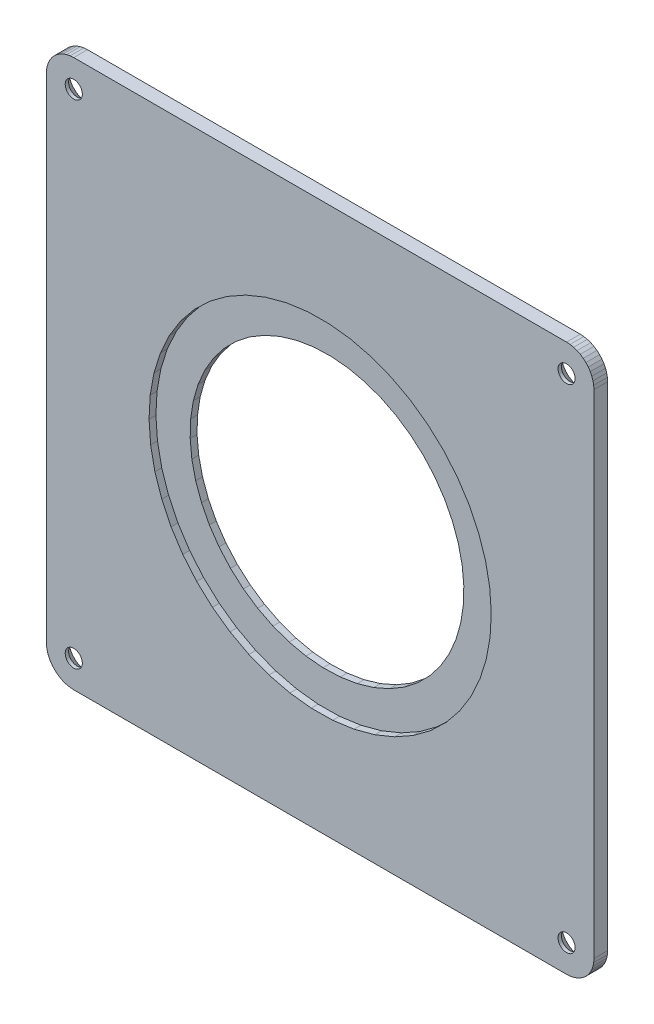
from build123d import *

# Parameters (mm, degrees)
BOSS_EXTRUDE1_DEPTH = 2.000000328
CUT_EXTRUDE1_DEPTH  = 57.60388554
CUT_EXTRUDE2_DEPTH  = 57.60388554
CUT_EXTRUDE3_DEPTH  = 57.60388554
CUT_EXTRUDE4_DEPTH  = 57.60388554
CUT_EXTRUDE5_DEPTH  = 0.999998301
CUT_EXTRUDE6_DEPTH  = 57.577379411
SKETCH9_R           = 2
CUT_EXTRUDE7_DEPTH  = 10
MOVE_FACE1_BY       = 0.75
MOVE_FACE1_2_BY     = 0.75
MOVE_FACE1_3_BY     = 0.75
MOVE_FACE1_4_BY     = 0.75
CHAMFER1_SIZE       = 1.5


with BuildPart() as part:
    # Sketch1 → Boss-Extrude1 (new body)
    with BuildSketch(Plane.XY.offset(37.080600858)):
        Polygon((-39.999999106, -35.99999845), (-39.965778589, -36.522105336), (-39.863705635, -37.035275251), (-39.695519954, -37.530735135), (-39.464101195, -37.999998778), (-39.173413068, -38.43504563), (-38.828425109, -38.828425109), (-38.43504563, -39.173413068), (-37.999998778, -39.464101195), (-37.530735135, -39.695519954), (-37.035275251, -39.863705635), (-36.522105336, -39.965778589), (-35.99999845, -39.999999106), (35.99999845, -39.999999106), (36.522105336, -39.965778589), (37.035275251, -39.863705635), (37.530735135, -39.695519954), (37.999998778, -39.464101195), (38.43504563, -39.173413068), (38.828425109, -38.828425109), (39.173413068, -38.43504563), (39.464101195, -37.999998778), (39.695519954, -37.530735135), (39.863705635, -37.035275251), (39.965778589, -36.522105336), (39.999999106, -35.99999845), (39.999999106, 35.99999845), (39.965778589, 36.522105336), (39.863705635, 37.035275251), (39.695519954, 37.530735135), (39.464101195, 37.999998778), (39.173413068, 38.43504563), (38.828425109, 38.828425109), (38.43504563, 39.173413068), (37.999998778, 39.464101195), (37.530735135, 39.695519954), (37.035275251, 39.863705635), (36.522105336, 39.965778589), (35.99999845, 39.999999106), (-35.99999845, 39.999999106), (-36.522105336, 39.965778589), (-37.035275251, 39.863705635), (-37.530735135, 39.695519954), (-37.999998778, 39.464101195), (-38.43504563, 39.173413068), (-38.828425109, 38.828425109), (-39.173413068, 38.43504563), (-39.464101195, 37.999998778), (-39.695519954, 37.530735135), (-39.863705635, 37.035275251), (-39.965778589, 36.522105336), (-39.999999106, 35.99999845), align=None)
    extrude(amount=-BOSS_EXTRUDE1_DEPTH)

    # Sketch2 → Cut-Extrude1 (cut, through all)
    with BuildSketch(Plane.XY.offset(37.080600858)):
        Polygon((-37.448886782, -36.388229579), (-37.29903698, -36.74999997), (-37.060663104, -37.060663104), (-36.74999997, -37.29903698), (-36.388229579, -37.448886782), (-35.99999845, -37.50000149), (-35.611771047, -37.448886782), (-35.250000656, -37.29903698), (-34.939337522, -37.060663104), (-34.700963646, -36.74999997), (-34.551113844, -36.388229579), (-34.499999136, -35.99999845), (-34.551113844, -35.611771047), (-34.700963646, -35.250000656), (-34.939337522, -34.939337522), (-35.250000656, -34.700963646), (-35.611771047, -34.551113844), (-35.99999845, -34.499999136), (-36.388229579, -34.551113844), (-36.74999997, -34.700963646), (-37.060663104, -34.939337522), (-37.29903698, -35.250000656), (-37.448886782, -35.611771047), (-37.50000149, -35.99999845), align=None)
    extrude(amount=-CUT_EXTRUDE1_DEPTH, mode=Mode.SUBTRACT)

    # Sketch3 → Cut-Extrude2 (cut, through all)
    with BuildSketch(Plane.XY.offset(37.080600858)):
        Polygon((-37.448886782, 35.611771047), (-37.29903698, 35.250000656), (-37.060663104, 34.939337522), (-36.74999997, 34.700963646), (-36.388229579, 34.551113844), (-35.99999845, 34.499999136), (-35.611771047, 34.551113844), (-35.250000656, 34.700963646), (-34.939337522, 34.939337522), (-34.700963646, 35.250000656), (-34.551113844, 35.611771047), (-34.499999136, 35.99999845), (-34.551113844, 36.388229579), (-34.700963646, 36.74999997), (-34.939337522, 37.060663104), (-35.250000656, 37.29903698), (-35.611771047, 37.448886782), (-35.99999845, 37.50000149), (-36.388229579, 37.448886782), (-36.74999997, 37.29903698), (-37.060663104, 37.060663104), (-37.29903698, 36.74999997), (-37.448886782, 36.388229579), (-37.50000149, 35.99999845), align=None)
    extrude(amount=-CUT_EXTRUDE2_DEPTH, mode=Mode.SUBTRACT)

    # Sketch4 → Cut-Extrude3 (cut, through all)
    with BuildSketch(Plane.XY.offset(37.080600858)):
        Polygon((34.787815064, -36.8835181), (35.057790577, -37.167146802), (35.391975194, -37.371244282), (35.767596215, -37.481889129), (35.99999845, -37.48762235), (36.159053327, -37.491546138), (36.539680178, -37.399572712), (36.88352638, -37.212212123), (37.167163198, -36.942245137), (37.371270724, -36.608066656), (37.481926864, -36.232448961), (37.491590859, -35.840992022), (37.399556488, -35.460323095), (37.212185562, -35.116482526), (36.942210048, -34.832850099), (36.608025432, -34.628756344), (36.232404411, -34.518111497), (35.840947181, -34.508455545), (35.460323095, -34.600444138), (35.116482526, -34.787815064), (34.832850099, -35.057790577), (34.628756344, -35.391975194), (34.518111497, -35.767596215), (34.508455545, -36.159053445), (34.600444138, -36.539677531), align=None)
    extrude(amount=-CUT_EXTRUDE3_DEPTH, mode=Mode.SUBTRACT)

    # Sketch5 → Cut-Extrude4 (cut, through all)
    with BuildSketch(Plane(origin=(0, 0, 35.08060053), x_dir=(-1, 0, 0), z_dir=(0, 0, -1))):
        Polygon((-36.388229579, 37.448886782), (-36.74999997, 37.29903698), (-37.060663104, 37.060663104), (-37.29903698, 36.74999997), (-37.448886782, 36.388229579), (-37.50000149, 35.99999845), (-37.448886782, 35.611771047), (-37.29903698, 35.250000656), (-37.060663104, 34.939337522), (-36.74999997, 34.700963646), (-36.388229579, 34.551113844), (-35.99999845, 34.499999136), (-35.611771047, 34.551113844), (-35.250000656, 34.700963646), (-34.939337522, 34.939337522), (-34.700963646, 35.250000656), (-34.551113844, 35.611771047), (-34.499999136, 35.99999845), (-34.551113844, 36.388229579), (-34.700963646, 36.74999997), (-34.939337522, 37.060663104), (-35.250000656, 37.29903698), (-35.611771047, 37.448886782), (-35.99999845, 37.50000149), align=None)
    extrude(amount=-CUT_EXTRUDE4_DEPTH, mode=Mode.SUBTRACT)

    # Sketch6 → Cut-Extrude5 (cut)
    with BuildSketch(Plane.XY.offset(37.080600858)):
        Polygon((-23.146180436, -9.447447956), (-21.779589355, -12.273938395), (-20.069517195, -14.906859957), (-18.042938784, -17.304692417), (-15.731809661, -19.429620355), (-13.172583655, -21.248130128), (-10.405616835, -22.73154445), (-7.474547718, -23.856470361), (-4.425600171, -24.605164304), (-1.306858379, -24.965818971), (1.832493464, -24.932749569), (4.94294567, -24.506473914), (7.975445129, -23.693718016), (10.882166214, -22.507296875), (13.617269695, -20.965922624), (16.137620434, -19.093904644), (18.403470516, -16.920762137), (20.379088819, -14.480772428), (22.033315152, -11.812409386), (23.34006317, -8.957758546), (24.278724566, -5.961838178), (24.834495038, -2.871896373), (24.998612702, 0.263337133), (24.768486619, 3.394417698), (24.147747084, 6.471966393), (23.146180436, 9.447447956), (21.779589355, 12.273938395), (20.069517195, 14.906859957), (18.042938784, 17.304692417), (15.731809661, 19.429620355), (13.172583655, 21.248130128), (10.405616835, 22.73154445), (7.474547718, 23.856470361), (4.425600171, 24.605164304), (1.306858379, 24.965818971), (-1.832493464, 24.932749569), (-4.94294567, 24.506473914), (-7.975445129, 23.693718016), (-10.882166214, 22.507296875), (-13.617269695, 20.965922624), (-16.137620434, 19.093904644), (-18.403470516, 16.920762137), (-20.379088819, 14.480772428), (-22.033315152, 11.812409386), (-23.34006317, 8.957758546), (-24.278724566, 5.961838178), (-24.834495038, 2.871896373), (-24.998612702, -0.263337133), (-24.768486619, -3.394417698), (-24.147747084, -6.471966393), align=None)
    extrude(amount=-CUT_EXTRUDE5_DEPTH, mode=Mode.SUBTRACT)

    # Sketch7 → Cut-Extrude6 (cut, through all)
    with BuildSketch(Plane.XY.offset(36.080602556)):
        Polygon((-19.744809717, -3.184724366), (-19.18996498, -5.634292495), (-18.332481384, -7.995004766), (-17.185883597, -10.229631327), (-15.768256038, -12.302929536), (-14.101952314, -14.182204381), (-12.213253416, -15.837816522), (-10.131943971, -17.243657261), (-7.89084658, -18.377555534), (-5.525306799, -19.221628085), (-3.072628984, -19.762564451), (-0.57149434, -19.991831854), (1.938653179, -19.905818626), (4.418227356, -19.50587891), (6.828122772, -18.79831776), (9.130334482, -17.794296145), (11.28855627, -16.509648412), (13.268750161, -14.964633621), (15.039687976, -13.183617964), (16.573440284, -11.194689199), (17.845820636, -9.029212408), (18.836760893, -6.721339654), (19.530635327, -4.30746749), (19.916500896, -1.825664192), (19.988268614, 0.684931001), (19.744809717, 3.184724366), (19.18996498, 5.634292495), (18.332481384, 7.995004766), (17.185883597, 10.229631327), (15.768256038, 12.302929536), (14.101952314, 14.182204381), (12.213253416, 15.837816522), (10.131943971, 17.243657261), (7.89084658, 18.377555534), (5.525306799, 19.221628085), (3.072628984, 19.762564451), (0.57149434, 19.991831854), (-1.938653179, 19.905818626), (-4.418227356, 19.50587891), (-6.828122772, 18.79831776), (-9.130334482, 17.794296145), (-11.28855627, 16.509648412), (-13.268750161, 14.964633621), (-15.039687976, 13.183617964), (-16.573440284, 11.194689199), (-17.845820636, 9.029212408), (-18.836760893, 6.721339654), (-19.530635327, 4.30746749), (-19.916500896, 1.825664192), (-19.988268614, -0.684931001), align=None)
    extrude(amount=-CUT_EXTRUDE6_DEPTH, mode=Mode.SUBTRACT)

    # Sketch9 → Cut-Extrude7 (cut)
    with BuildSketch(Plane(origin=(0, 0, 35.08060053), x_dir=(-1, 0, 0), z_dir=(0, 0, -1))):
        with Locations((35.99999845, 35.99999845)):
            Circle(SKETCH9_R)
        with Locations(Location((35.99999845, -35.99999845, 0), (0, 0, 180))):
            Circle(SKETCH9_R)
        with Locations((-35.99999845, -35.99999845)):
            Circle(SKETCH9_R)
        with Locations(Location((-35.99999845, 35.99999845, 0), (0, 0, 180))):
            Circle(SKETCH9_R)
    extrude(amount=-CUT_EXTRUDE7_DEPTH, mode=Mode.SUBTRACT)

    # Move Face1: a curved face moved outward by 0.75
    add(Solid.thicken(part.faces().sort_by_distance((33.99999845, 35.99999845, 36.080600694))[0], MOVE_FACE1_BY))

    # Move Face1 2: a curved face moved outward by 0.75
    add(Solid.thicken(part.faces().sort_by_distance((37.99999845, -35.99999845, 36.080600694))[0], MOVE_FACE1_2_BY))

    # Move Face1 3: a curved face moved outward by 0.75
    add(Solid.thicken(part.faces().sort_by_distance((-37.99999845, -35.99999845, 36.080600694))[0], MOVE_FACE1_3_BY))

    # Move Face1 4: a curved face moved outward by 0.75
    add(Solid.thicken(part.faces().sort_by_distance((-33.99999845, 35.99999845, 36.080600694))[0], MOVE_FACE1_4_BY))

    # Chamfer1
    chamfer1_edges = [part.edges().sort_by_distance(p)[0] for p in [
        (34.74999845, 35.99999845, 35.08060053),
        (37.24999845, -35.99999845, 35.08060053),
        (-37.24999845, -35.99999845, 35.08060053),
        (-34.74999845, 35.99999845, 35.08060053),
    ]]
    chamfer(chamfer1_edges, length=CHAMFER1_SIZE)


solid = part.part
